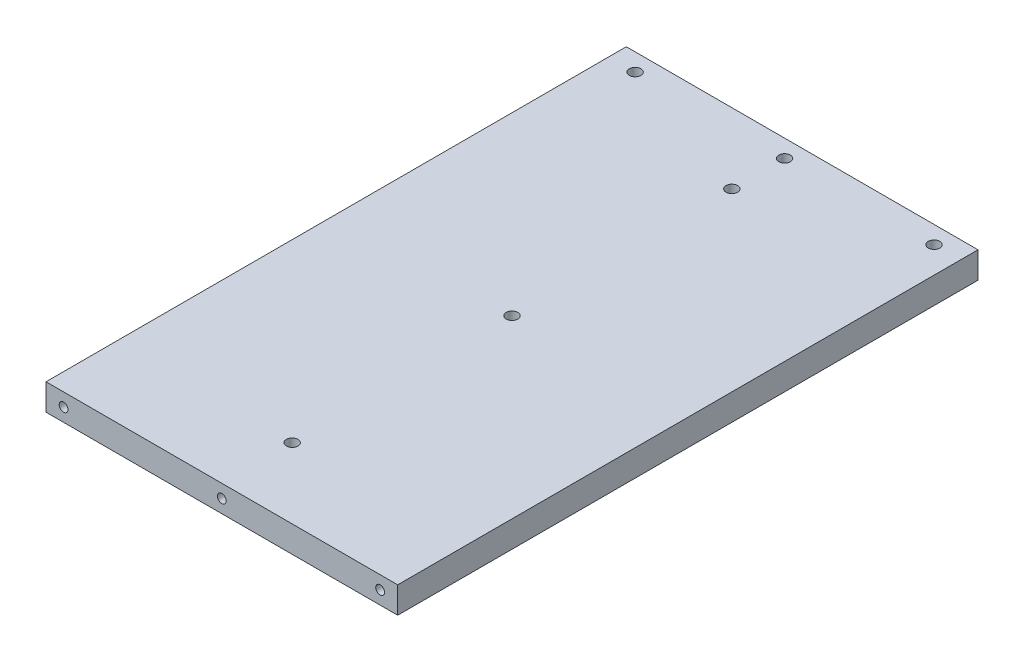
SolidWorks part; units mm, degrees
material "6061"
ref_plane "前视基准面" through (0, 0, 0) normal (0, 0, 1) x (1, 0, 0)
ref_plane "上视基准面" through (0, 0, 0) normal (0, 1, 0) x (1, 0, 0)
ref_plane "右视基准面" through (0, 0, 0) normal (1, 0, 0) x (0, 0, -1)
sketch "草图1" plane through (0, 0, 0) normal (0, 1, 0) x (1, 0, 0)
  line L1 (100, -165) -> (-100, -165)
  line L2 (100, -165) -> (100, 165)
  line L3 (100, 165) -> (-100, 165)
  line L4 (-100, -165) -> (-100, 165)
  line L5 (100, -165) -> (-100, 165) construction
  line L6 (100, 165) -> (-100, -165) construction
  point P0 (0, 0)
  dimension "D1" = 200
  dimension "D2" = 330
extrude "凸台-拉伸1" add sketch "草图1" along normal mid plane 15
hole_wizard "M6 六角凹头螺钉的柱形沉头孔1" positions "草图2" profile "草图3" counterbore size "M6" standard "ISO" end condition through all
sketch "草图2" plane through (0, -7.5, 0) normal (0, -1, 0) x (-1, 0, 0)
  line L0 (0, -165) -> (0, 192.6016) construction
  line L1 (100, -165) -> (-100, -165) construction
  line L3 (100, 0) -> (-118.4809, 0) construction
  line L4 (100, 165) -> (100, -165) construction
  point P0 (0, 0)
  point P3 (0, -125)
  point P5 (0, 125)
  dimension "D1" = 250
sketch "草图3" plane through (0, -7.5, 0) normal (1, 0, 0) x (0, 0, -1)
  line L0 (0, 0) -> (0, 15)
  line L1 (0, 15) -> (3.3, 15)
  line L3 (3.3, 15) -> (3.3, 8)
  line L4 (3.3, 8) -> (5.5, 8)
  line L5 (5.5, 8) -> (5.5, 0)
  line L7 (5.5, 0) -> (0, 0)
  line L11 (0, -6.35) -> (0, 107.95) construction
  dimension "通孔孔直径" = 6.6
  dimension "通孔孔深度" = 15
  dimension "柱形沉头孔直径" = 11
  dimension "柱形沉头孔深度" = 8
hole_wizard "M6 六角凹头螺钉的柱形沉头孔2" positions "草图4" profile "草图5" counterbore size "M6" standard "ISO" end condition through all
sketch "草图4" plane through (0, -7.5, 0) normal (0, -1, 0) x (-1, 0, 0)
  line L0 (100, 155) -> (-100, 155) construction
  line L1 (100, 165) -> (100, -165) construction
  line L2 (-100, -165) -> (-100, 165) construction
  line L4 (-100, 165) -> (100, 165) construction
  line L5 (0, -165) -> (0, 298.5695) construction
  line L6 (100, -165) -> (-100, -165) construction
  point P0 (85, 155)
  point P2 (0, 155)
  point P4 (-85, 155)
  dimension "D1" = 10
  dimension "D2" = 170
sketch "草图5" plane through (-85, -7.5, -155) normal (1, 0, 0) x (0, 0, -1)
  line L0 (0, 0) -> (0, 15)
  line L1 (0, 15) -> (3.3, 15)
  line L3 (3.3, 15) -> (3.3, 8)
  line L4 (3.3, 8) -> (5.5, 8)
  line L5 (5.5, 8) -> (5.5, 0)
  line L7 (5.5, 0) -> (0, 0)
  line L11 (0, -6.35) -> (0, 107.95) construction
  dimension "通孔孔直径" = 6.6
  dimension "通孔孔深度" = 15
  dimension "柱形沉头孔直径" = 11
  dimension "柱形沉头孔深度" = 8
hole_wizard "M6 螺纹孔1" positions "草图6" profile "草图7" tap size "M6" standard "ISO"
sketch "草图6" plane through (0, 0, 165) normal (0, 0, 1) x (1, 0, 0)
  point P0 (0, 0)
  point P3 (-90, 0)
  point P6 (90, 0)
sketch "草图7" plane through (0, 0, 165) normal (1, 0, 0) x (0, -1, 0)
  line L0 (0, 0) -> (0, 18.5022)
  line L1 (0, 18.5022) -> (2.5, 17)
  line L2 (2.5, 17) -> (2.5, 0)
  line L5 (2.5, 0) -> (0, 0)
  line L10 (0, 18.5022) -> (-2.5, 17) construction
  line L11 (0, -6.35) -> (0, 107.95) construction
  dimension "螺纹孔钻头直径" = 5
  dimension "螺纹孔钻头深度" = 17
  dimension "导头角度" = 118
cosmetic thread "孔螺蚊线1"
cosmetic thread "孔螺蚊线3"
cosmetic thread "孔螺蚊线4"
